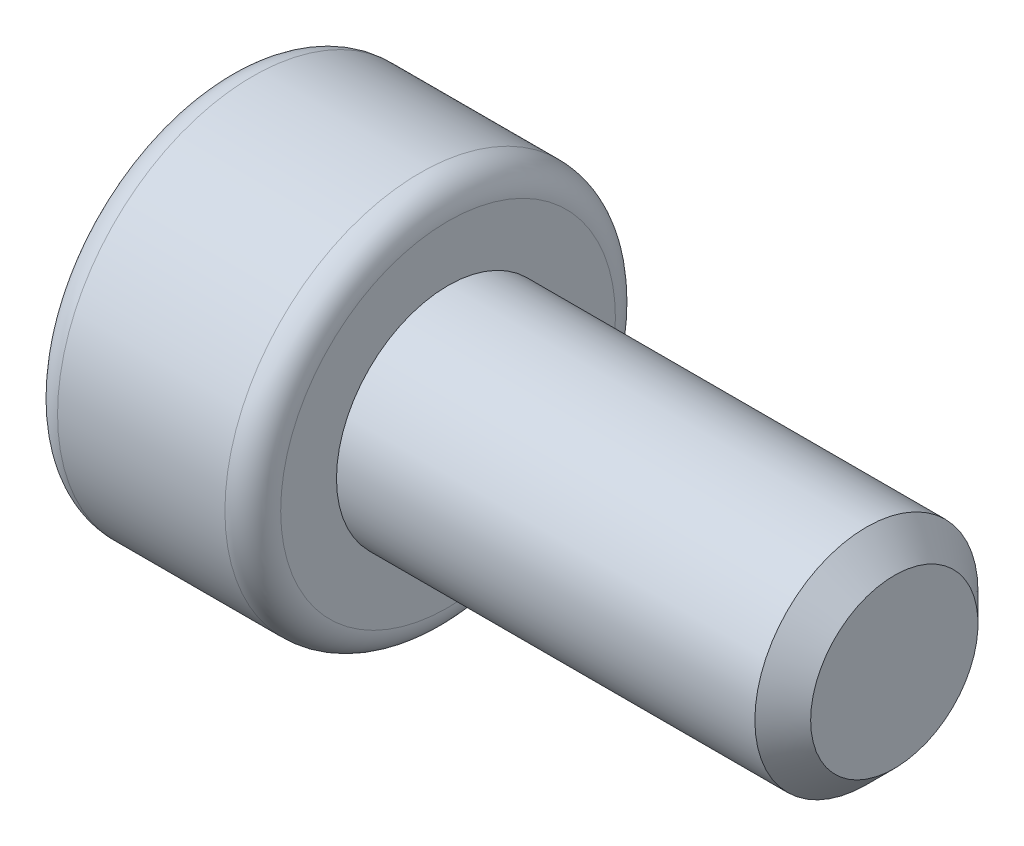
from build123d import *

# Parameters (mm, degrees)
CUT_EXTRUDE1_DEPTH = 2
FILLET1_R          = 0.5
CHAMFER1_SIZE      = 0.1
CHAMFER1_SIZE2     = 0.567128182
CHAMFER2_SIZE      = 0.5


with BuildPart() as part:
    # Sketch1 → Revolve1 (revolve)
    with BuildSketch(Plane.XY, mode=Mode.PRIVATE) as revolve1_sk:
        Polygon((0, 0), (0, 3.5), (4, 3.5), (4, 2), (12, 2), (12, 0), align=None)
    revolve(revolve1_sk.sketch.rotate(Axis((-4.709244637, 0, 0), (1, 0, 0)), 90), axis=Axis((-4.709244637, 0, 0), (1, 0, 0)))

    # Sketch4 → Cut-Extrude1 (cut)
    with BuildSketch(Plane.ZY):
        Polygon((-1.732050808, 0), (-0.866025404, -1.5), (0.866025404, -1.5), (1.732050808, 0), (0.866025404, 1.5), (-0.866025404, 1.5), align=None)
    extrude(amount=-CUT_EXTRUDE1_DEPTH, mode=Mode.SUBTRACT)

    # Fillet1
    fillet1_edges = [part.edges().sort_by_distance(p)[0] for p in [
        (4, 0, -3.5),
        (0, 0, -3.5),
    ]]
    fillet(fillet1_edges, radius=FILLET1_R)

    # Chamfer1
    chamfer1_edges = [part.edges().sort_by_distance(p)[0] for p in [
        (0, 0.75, -1.299038106),
        (0, -0.75, -1.299038106),
        (0, -1.5, 0),
        (0, -0.75, 1.299038106),
        (0, 0.75, 1.299038106),
        (0, 1.5, 0),
    ]]
    chamfer1_side = [part.faces().sort_by_distance(p)[0] for p in [
        (0, 0, -2.915147186),
    ]]
    chamfer(chamfer1_edges, length=CHAMFER1_SIZE, length2=CHAMFER1_SIZE2, reference=chamfer1_side[0])

    # Chamfer2
    chamfer2_edges = [part.edges().sort_by_distance(p)[0] for p in [
        (12, 0, -2),
    ]]
    chamfer(chamfer2_edges, length=CHAMFER2_SIZE)


solid = part.part
